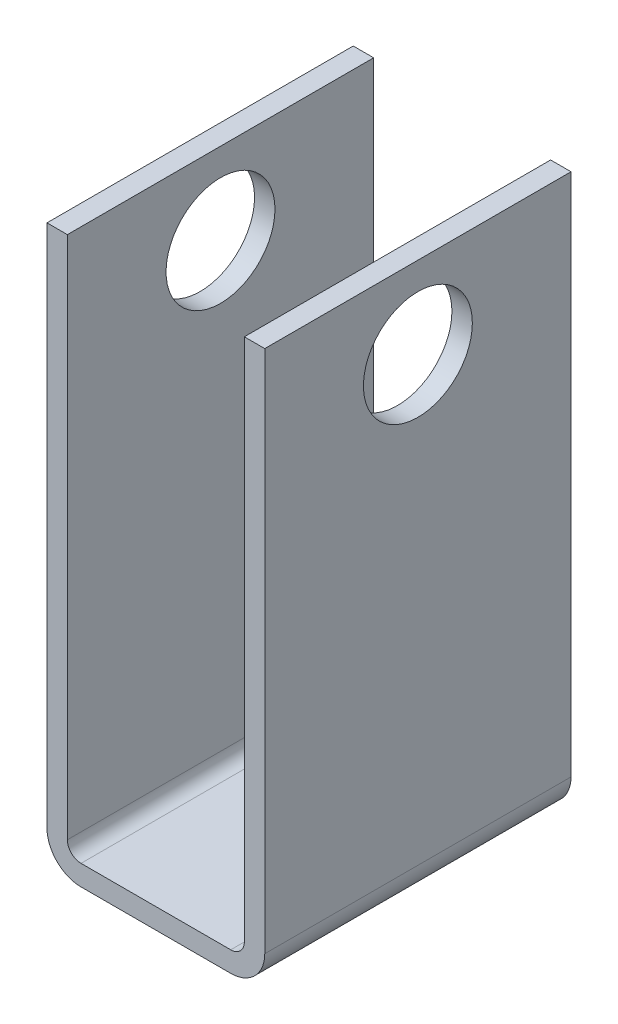
from build123d import *

# Parameters (mm, degrees)
BOSS_EXTRUDE1_DEPTH = 45
SKETCH2_R           = 8
CUT_EXTRUDE1_DEPTH  = 99.858484714


with BuildPart() as part:
    # Sketch1 → Boss-Extrude1 (new body)
    with BuildSketch(Plane.XY):
        with BuildLine():
            Line((0, 0), (0, -77))
            ThreePointArc((0, -77), (1.464466094, -80.535533906), (5, -82))
            Line((5, -82), (27, -82))
            ThreePointArc((27, -82), (30.535533906, -80.535533906), (32, -77))
            Line((32, -77), (32, 0))
            Line((32, 0), (29, 0))
            Line((29, 0), (29, -77))
            ThreePointArc((29, -77), (28.414213562, -78.414213562), (27, -79))
            Line((27, -79), (5, -79))
            ThreePointArc((5, -79), (3.585786438, -78.414213562), (3, -77))
            Line((3, -77), (3, 0))
            Line((3, 0), (0, 0))
        make_face()
    extrude(amount=BOSS_EXTRUDE1_DEPTH)

    # Sketch2 → Cut-Extrude1 (cut, through all)
    with BuildSketch(Plane(origin=(32, 0, 0), x_dir=(0, 0, -1), z_dir=(1, 0, 0))):
        with Locations((-22.5, -12)):
            Circle(SKETCH2_R)
    extrude(amount=-CUT_EXTRUDE1_DEPTH, mode=Mode.SUBTRACT)


solid = part.part
